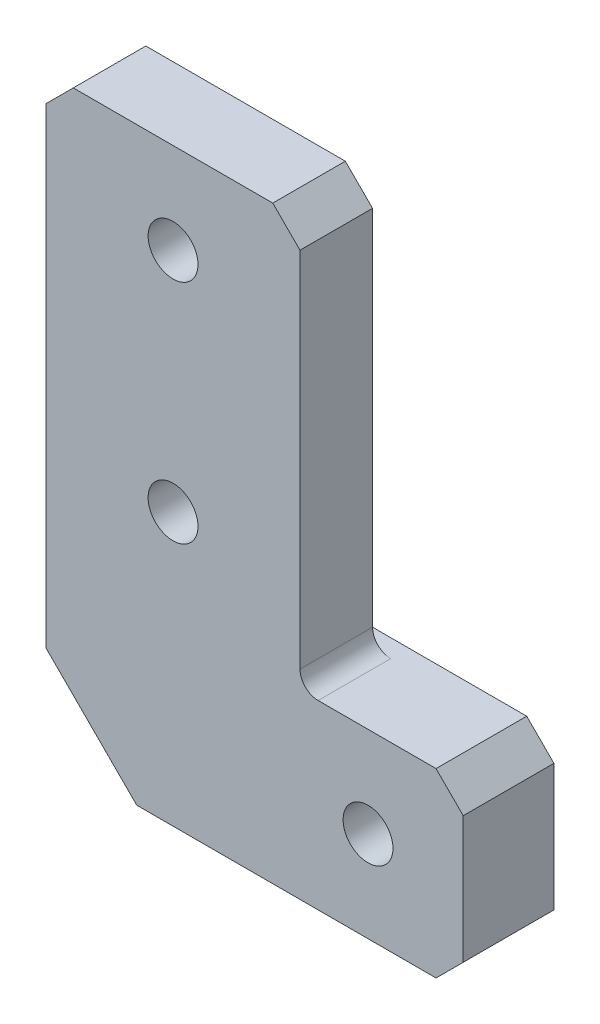
SolidWorks part; units mm, degrees
ref_plane "Front Plane" through (0, 0, 0) normal (0, 0, 1) x (1, 0, 0)
ref_plane "Top Plane" through (0, 0, 0) normal (0, 1, 0) x (1, 0, 0)
ref_plane "Right Plane" through (0, 0, 0) normal (1, 0, 0) x (0, 0, -1)
sketch "Sketch1" plane through (0, 0, 0) normal (0, 0, 1) x (1, 0, 0)
  line L1 (0, 0) -> (-46, 0)
  line L2 (0, 0) -> (0, 65)
  line L3 (0, 65) -> (-46, 65)
  line L4 (-46, 0) -> (-46, 65)
  dimension "D1" = 46
  dimension "D2" = 65
extrude "Boss-Extrude1" add sketch "Sketch1" along normal blind 8
sketch "Sketch2" plane through (0, 0, 8) normal (0, 0, 1) x (1, 0, 0)
  line L0 (0, 0) -> (0, 65) construction
  line L1 (-46, 0) -> (0, 0) construction
  circle A0 centre (-10.5, 10) radius 2.75
  dimension "D1" = 5.5
  dimension "D2" = 10.5
  dimension "D3" = 10
extrude "Cut-Extrude1" cut sketch "Sketch2" against normal blind 18
chamfer "Chamfer1" distance 10 angle 45 1 edges at (-46, 0, 4)
sketch "Sketch3" plane through (0, 0, 8) normal (0, 0, 1) x (1, 0, 0)
  line L1 (0, 65) -> (-46, 65) construction
  line L2 (-46, 65) -> (-46, 10) construction
  circle A0 centre (-32, 55) radius 2.75
  circle A1 centre (-32, 30) radius 2.75
  dimension "D1" = 5.5
  dimension "D2" = 14
  dimension "D3" = 25
  dimension "D4" = 10
extrude "Cut-Extrude2" cut sketch "Sketch3" against normal blind 10
sketch "Sketch4" plane through (0, 0, 8) normal (0, 0, 1) x (1, 0, 0)
  line L0 (-46, 65) -> (-46, 10) construction
  line L1 (0, 65) -> (-18, 65)
  line L2 (0, 65) -> (0, 20)
  line L3 (0, 20) -> (-18, 20)
  line L4 (-18, 65) -> (-18, 20)
  dimension "D1" = 28
  dimension "D2" = 45
extrude "Cut-Extrude3" cut sketch "Sketch4" against normal blind 10
sketch "Sketch5" plane through (0, 0, 0) normal (0, 0, -1) x (-1, 0, 0)
  line L0 (46, 65) -> (46, 10) construction
  line L1 (0, 20) -> (46, 20)
  line L2 (0, 20) -> (0, 0)
  line L5 (36, 0) -> (46, 10) construction
  line L6 (36, 0) -> (0, 0) construction
  line L7 (46, 20) -> (46, 10)
  line L8 (36, 0) -> (46, 10)
  line L9 (36, 0) -> (0, 0)
  circle A0 centre (10.5, 10) radius 2.75 construction
  circle A1 centre (10.5, 10) radius 2.75
extrude "Boss-Extrude2" add sketch "Sketch5" along normal blind 2
fillet "Fillet1" radius 2 1 edges
chamfer "Chamfer2" distance 3 angle 45 4 edges at (0, 0, 3) (0, 20, 3) (-18, 65, 4) (-46, 65, 4)
